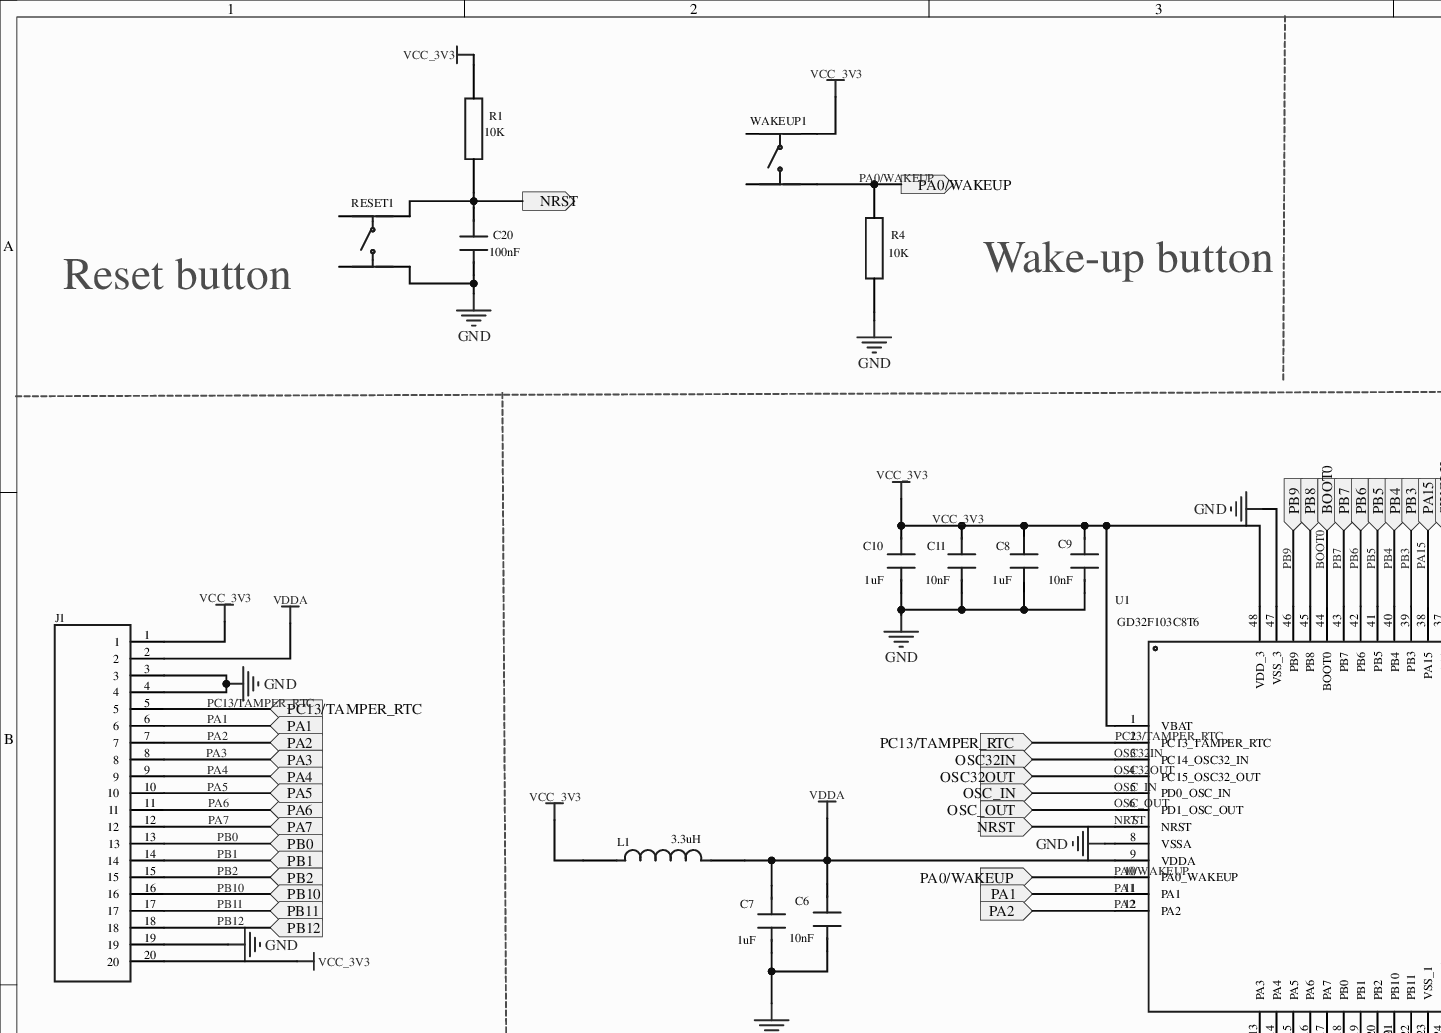
[diagram p0: MISC50188-3.schdoc, top left]
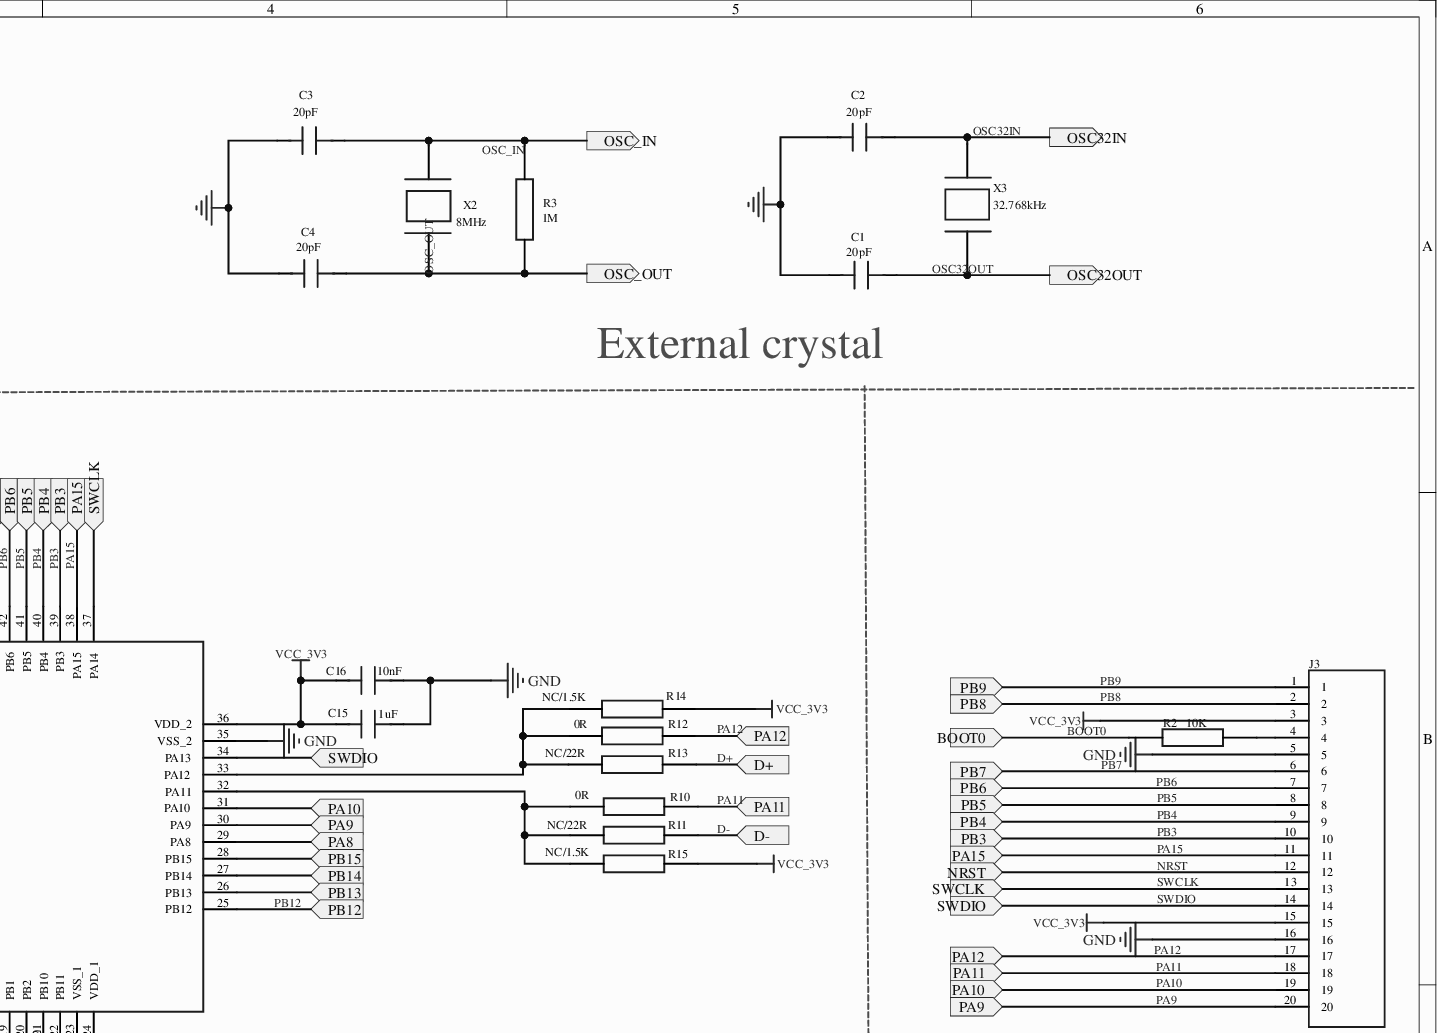
[diagram p1: MISC50188-3.schdoc, top right]
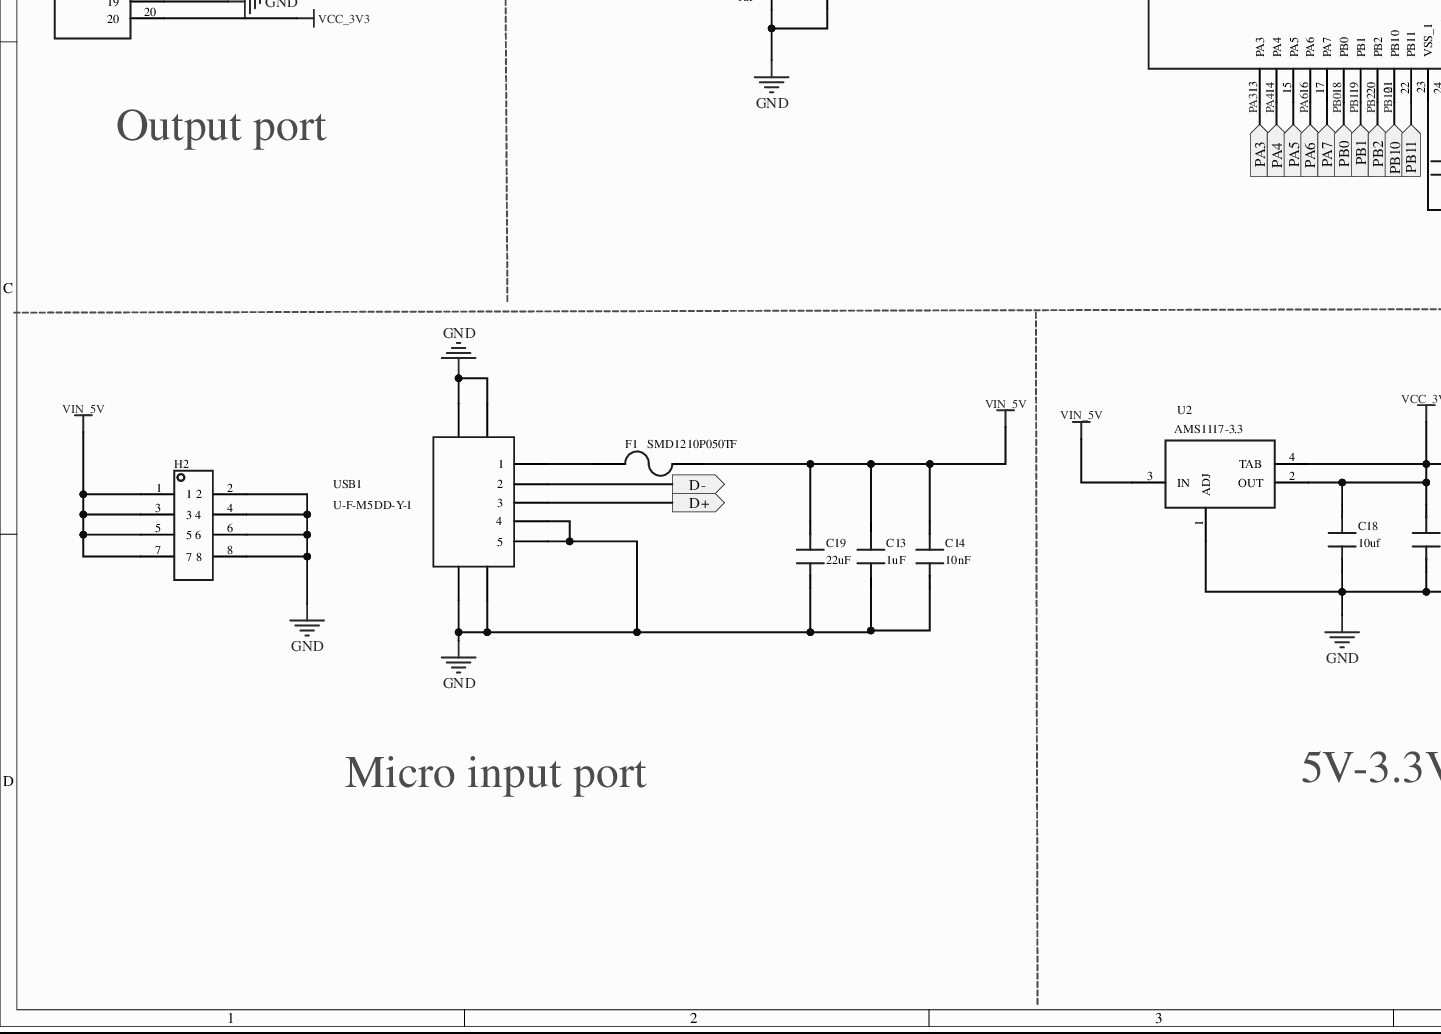
[diagram p2: MISC50188-3.schdoc, bottom left]
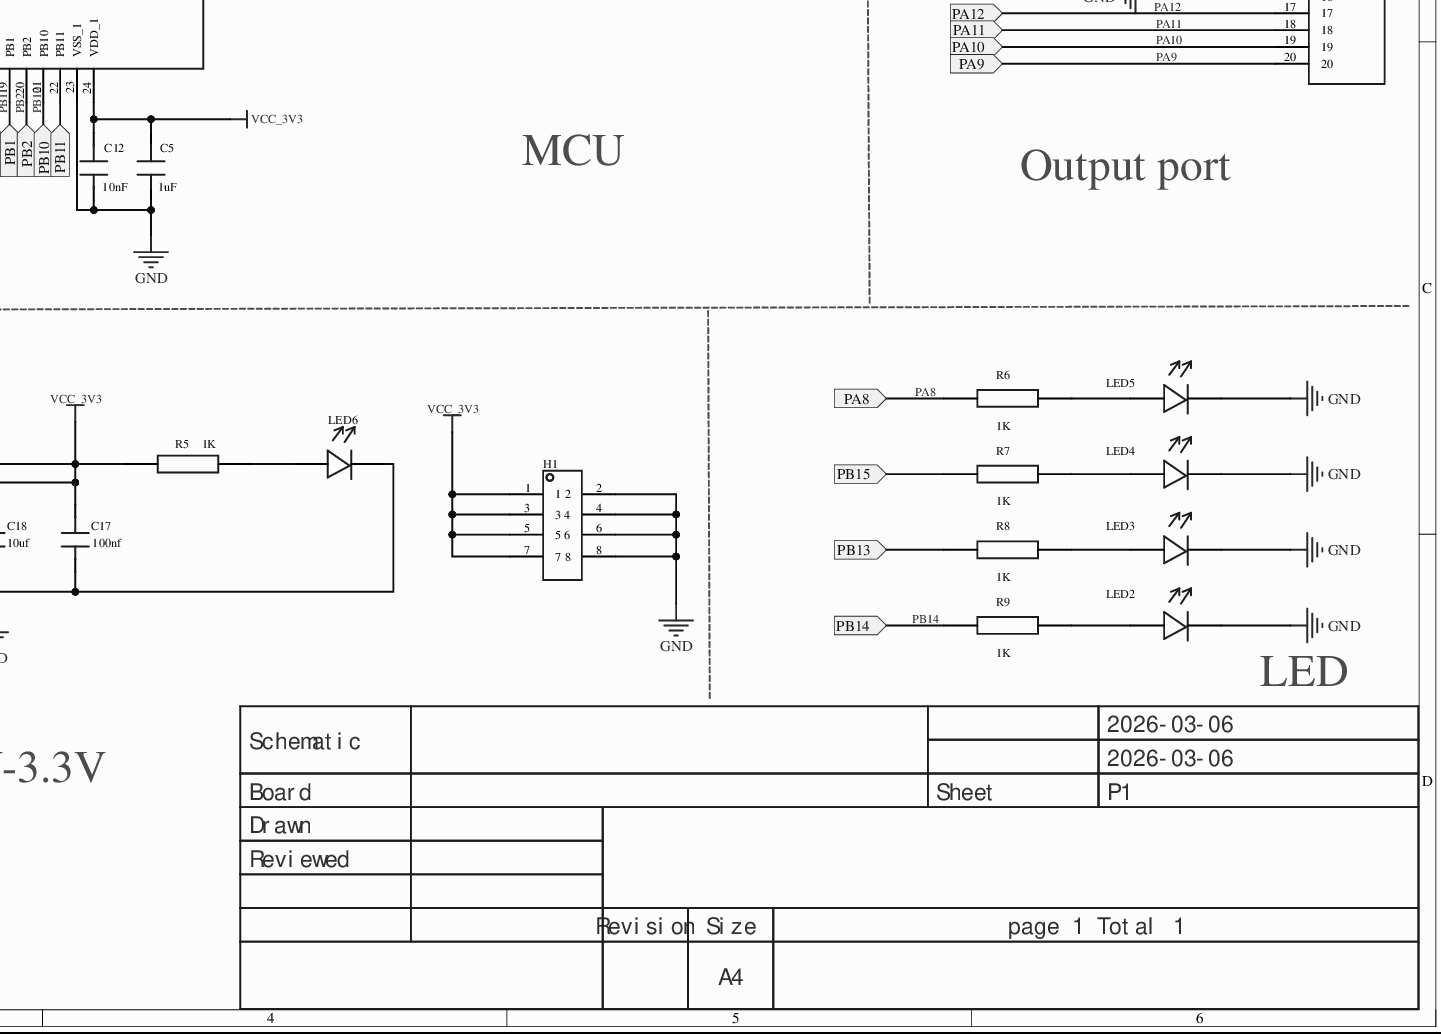
[diagram p3: MISC50188-3.schdoc, bottom right]
# Altium project MISC50188-2.PrjPcb
1 sheet, 53 parts. Net scope: flat (ports and power ports of the same name join across sheets).
Board file: MISC50188.pcbdoc

## Sheet MISC50188-3.schdoc
size 420 x 297 mm; Version: V1.0; @Project Name: MISC50188; @Page Count: 1; @Update Date: 2026-03-06; @Create Date: 2026-03-06; @Schematic Name: MISC50188; @Page No: 1; @Board Name: MISC50188; @Create Time: 01:33:52; @Update Time: 21:43:49; Size: A4

### Parts
C1  20pF  [C0603]
C2  20pF  [C0603]
C3  20pF  [C0603]
C4  20pF  [C0603]
C5  1uF  [C0603]
C6  10nF  [C0603]
C7  1uF  [C0603]
C8  1uF  [C0603]
C9  10nF  [C0603]
C10  1uF  [C0603]
C11  10nF  [C0603]
C12  10nF  [C0603]
C13  1uF  [C0603]
C14  10nF  [C0603]
C15  1uF  [C0603]
C16  10nF  [C0603]
C17  100nf  [C0603]
C18  10uf  [C0805]
C19  22uF  [C0805]
C20  100nF  [C0603]
F1  (no value)  [F1210]
H1  (no value)  [HDR-TH_8P-P2.54-V-M-R2-C4-S2.54]
H2  (no value)  [HDR-TH_8P-P2.54-V-M-R2-C4-S2.54]
J1  (no value)  [HDR-TH_20PIN-V-MALE-PITCH2.54]
J3  (no value)  [HDR-TH_20PIN-V-MALE-PITCH2.54]
L1  3.3uH  [L0603]
LED2  (no value)  [LED0603]
LED3  (no value)  [LED0603]
LED4  (no value)  [LED0603]
LED5  (no value)  [LED0603]
LED6  (no value)  [LED0603]
R1  10K  [R0603]
R2  10K  [R0603]
R3  1M  [R0603]
R4  10K  [R0603]
R5  1K  [R0603]
R6  1K  [R0603]
R7  1K  [R0603]
R8  1K  [R0603]
R9  1K  [R0603]
R10  0R  [R0603]
R11  NC/22R  [R0603]
R12  0R  [R0603]
R13  NC/22R  [R0603]
R14  NC/1.5K  [R0603]
R15  NC/1.5K  [R0603]
RESET1  (no value)  [SW-SMD-T6X6-9.5X5.8]
U1  (no value)  [TQFP-48_L7.0-W7.0-P0.50-LS9.0-BL]
U2  (no value)  [SOT-223]
USB1  (no value)  [U-F-M5DD-Y-1]
WAKEUP1  (no value)  [SW-SMD-T6X6-9.5X5.8]
X2  8MHz  [OSC-49S-1]
X3  32.768kHz  [DT-38_BD3.1-P0.80]

### Ports
BOOT0 (in), D+ (in), D+ (out), D- (in), D- (out), NRST (in), NRST (out), OSC32IN (in), OSC32IN (out), OSC32OUT (in), OSC32OUT (out), OSC_IN (in), OSC_IN (out), OSC_OUT (in), OSC_OUT (out), PA0/WAKEUP (in), PA0/WAKEUP (out), PA1 (in), PA2 (in), PA3 (in), PA4 (in), PA5 (in), PA6 (in), PA7 (in), PA8 (in), PA9 (in), PA10 (in), PA11 (in), PA12 (in), PA15 (in), PB0 (in), PB1 (in), PB2 (in), PB3 (in), PB4 (in), PB5 (in), PB6 (in), PB7 (in), PB8 (in), PB9 (in), PB10 (in), PB11 (in), PB12 (in), PB13 (in), PB14 (in), PB15 (in), PC13/TAMPER_RTC (in), SWCLK (in), SWDIO (in)

### Nets
GND: C1.1 C2.1 C3.1 C4.1 C5.1 C6.1 C7.1 C8.1 C9.1 C10.1 C11.1 C12.1 C13.1 C14.1 C15.2 C16.2 C17.1 C18.1 C19.1 C20.1 H1.2 H1.4 H1.6 H1.8 H2.2 H2.4 H2.6 H2.8 J1.3 J1.4 J1.19 J3.5 J3.16 LED2.1 LED3.1 LED4.1 LED5.1 LED6.1 R4.1(R-) RESET1.3 U1.8(VSSA) U1.23(VSS_1) U1.35(VSS_2) U1.47(VSS_3) U2.1(ADJ) USB1.4 USB1.5 USB1.6 USB1.7 USB1.8 USB1.9
VCC_3V3: C5.2 C8.2 C9.2 C10.2 C11.2 C12.2 C15.1 C16.1 C17.2 C18.2 H1.1 H1.3 H1.5 H1.7 J1.1 J1.20 J3.3 J3.15 L1.1 R1.2(R+) R5.1(R-) R14.2(R+) R15.2(R+) U1.1(VBAT) U1.24(VDD_1) U1.36(VDD_2) U1.48(VDD_3) U2.2(OUT) U2.4(TAB) WAKEUP1.1
VDDA: C6.2 C7.2 J1.2 L1.2 U1.9(VDDA)
VIN_5V: C13.2 C14.2 C19.2 F1.2 H2.1 H2.3 H2.5 H2.7 U2.3(IN)
BOOT0: R2.1(R-) U1.44(BOOT0) ; port BOOT0
D+: R13.2(R+) USB1.3 ; port D+
D-: R11.2(R+) USB1.2 ; port D-
NRST: C20.2 J3.12 R1.1(R-) RESET1.1 U1.7(NRST) ; port NRST
OSC32IN: C2.2 U1.3(PC14_OSC32_IN) X3.1 ; port OSC32IN
OSC32OUT: C1.2 U1.4(PC15_OSC32_OUT) X3.2 ; port OSC32OUT
OSC_IN: C3.2 R3.2(R+) U1.5(PD0_OSC_IN) X2.2 ; port OSC_IN
OSC_OUT: C4.2 R3.1(R-) U1.6(PD1_OSC_OUT) X2.1 ; port OSC_OUT
PA0/WAKEUP: R4.2(R+) U1.10(PA0_WAKEUP) WAKEUP1.3 ; port PA0/WAKEUP
PA1: J1.6 U1.11(PA1) ; port PA1
PA2: J1.7 U1.12(PA2) ; port PA2
PA3: J1.8 U1.13(PA3) ; port PA3
PA4: J1.9 U1.14(PA4) ; port PA4
PA5: J1.10 U1.15(PA5) ; port PA5
PA6: J1.11 U1.16(PA6) ; port PA6
PA7: J1.12 U1.17(PA7) ; port PA7
PA8: R6.1(R-) U1.29(PA8) ; port PA8
PA9: J3.20 U1.30(PA9) ; port PA9
PA10: J3.19 U1.31(PA10) ; port PA10
PA11: J3.18 R10.2(R+) ; port PA11
PA12: J3.17 R12.2(R+) ; port PA12
PA15: J3.11 U1.38(PA15) ; port PA15
PB0: J1.13 U1.18(PB0) ; port PB0
PB1: J1.14 U1.19(PB1) ; port PB1
PB2: J1.15 U1.20(PB2) ; port PB2
PB3: J3.10 U1.39(PB3) ; port PB3
PB4: J3.9 U1.40(PB4) ; port PB4
PB5: J3.8 U1.41(PB5) ; port PB5
PB6: J3.7 U1.42(PB6) ; port PB6
PB7: J3.6 U1.43(PB7) ; port PB7
PB8: J3.2 U1.45(PB8) ; port PB8
PB9: J3.1 U1.46(PB9) ; port PB9
PB10: J1.16 U1.21(PB10) ; port PB10
PB11: J1.17 U1.22(PB11) ; port PB11
PB12: J1.18 U1.25(PB12) ; port PB12
PB14: R9.1(R-) U1.27(PB14) ; port PB14
PC13/TAMPER_RTC: J1.5 U1.2(PC13_TAMPER_RTC) ; port PC13/TAMPER_RTC
SWCLK: J3.13 U1.37(PA14) ; port SWCLK
SWDIO: J3.14 U1.34(PA13) ; port SWDIO
NetF1_1: F1.1 USB1.1
NetJ3_4: J3.4 R2.2(R+)
NetLED2_2: LED2.2 R9.2(R+)
NetLED3_2: LED3.2 R8.2(R+)
NetLED4_2: LED4.2 R7.2(R+)
NetLED5_2: LED5.2 R6.2(R+)
NetLED6_2: LED6.2 R5.2(R+)
NetR7_1: R7.1(R-) U1.28(PB15) ; port PB15
NetR8_1: R8.1(R-) U1.26(PB13) ; port PB13
NetR10_1: R10.1(R-) R11.1(R-) R15.1(R-) U1.32(PA11)
NetR12_1: R12.1(R-) R13.1(R-) R14.1(R-) U1.33(PA12)

Not connected (* = marked no-connect by the designer): RESET1 2* 4*; WAKEUP1 2* 4*

### Notes on the sheet
- (near RESET1) Reset button
- Wake-up button
- (near C1) External crystal
- Output port
- MCU
- LED
- Micro input port
- 5V-3.3V
- 2026-03-06
- Schematic
- Board
- Sheet
- P1
- Drawn
- Reviewed
- Revision
- Size
- A4
- page 1 Total 1

### Library data of the parts
C1-C20 = C: AddInBom: yes; Device: C; SymbolName: C; ConvertToPcb: yes
F1 = SMD1210P050TF: AddInBom: yes; Device: SMD1210P050TF; SymbolName: SMD1210P050TF; ConvertToPcb: yes
H1 H2 = PZ254V-12-8P: AddInBom: yes; Device: PZ254V-12-8P; SymbolName: PZ254V-12-8P; ConvertToPcb: yes
J1 J3 = HDR-20P: AddInBom: yes; Device: HDR-20P; SymbolName: HDR-20P; ConvertToPcb: yes
L1 = L: AddInBom: yes; Device: L; SymbolName: 3.3uH; ConvertToPcb: yes
LED2-LED6 = LED: AddInBom: yes; Device: LED; SymbolName: LED; ConvertToPcb: yes
R1-R15 = R: Resistor; AddInBom: yes; Device: R; SymbolName: R; ConvertToPcb: yes
RESET1 WAKEUP1 = TSA063G43-250: AddInBom: yes; Device: TSA063G43-250; SymbolName: TSA063G43-250; ConvertToPcb: yes
U1 = GD32F103C8T6: AddInBom: yes; Device: GD32F103C8T6; SymbolName: GD32F103C8T6; ConvertToPcb: yes
U2 = AMS1117-3.3: AddInBom: yes; Device: AMS1117-3.3; SymbolName: AMS1117-3.3; ConvertToPcb: yes
USB1 = U-F-M5DD-Y-1: AddInBom: yes; Device: U-F-M5DD-Y-1; SymbolName: U-F-M5DD-Y-1; ConvertToPcb: yes
X2 X3 = 晶振: Device: Crystal oscillator; AddInBom: yes; SymbolName: Crystal oscillator; ConvertToPcb: yes